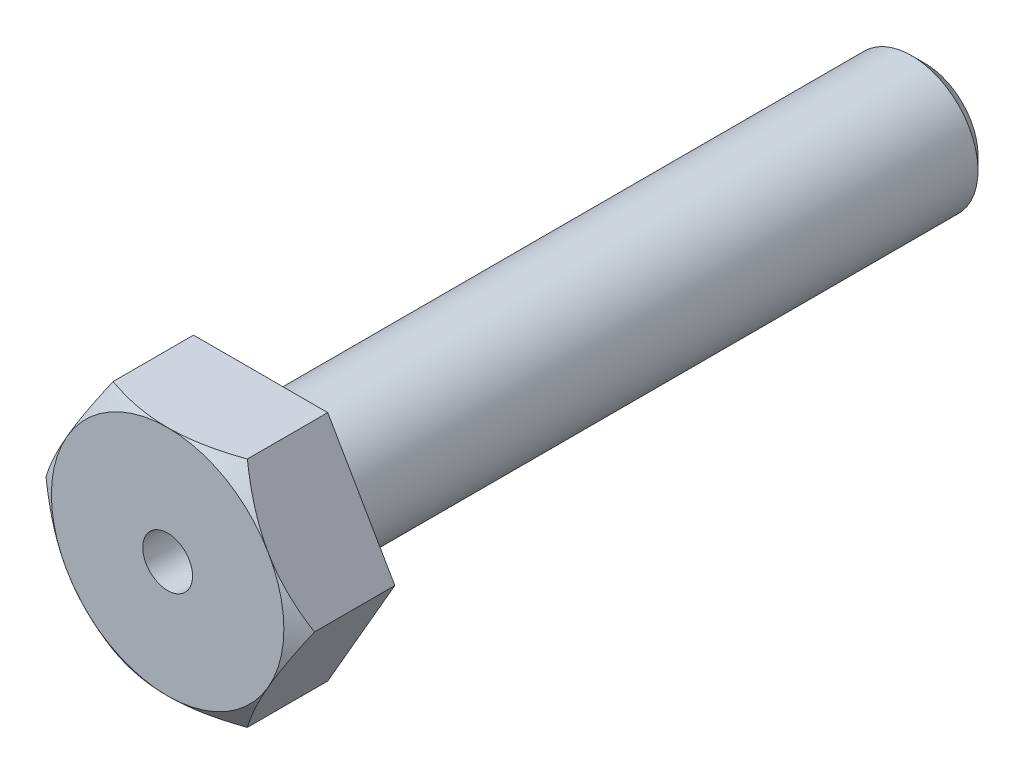
from build123d import *

# Parameters (mm, degrees)
BOSS_EXTRUDE1_START = -2.8
SKETCH4_R           = 0.75
BOSS_EXTRUDE1_DEPTH = 2.8
SKETCH5_R           = 4.582903769
SKETCH5_R_2         = 3.5
CUT_EXTRUDE1_DEPTH  = 1
CUT_EXTRUDE1_DRAFT  = -55
CHAMFER1_SIZE       = 0.4


with BuildPart() as part:
    # Sketch3 → Revolve1 (revolve)
    with BuildSketch(Plane(origin=(0, 0, 0), x_dir=(0, 0, -1), z_dir=(1, 0, 0)), mode=Mode.PRIVATE) as revolve1_sk:
        Polygon((0, 2), (-2.8, 2), (-2.8, 0.75), (20, 0.75), (20, 2), align=None)
    revolve(revolve1_sk.sketch.rotate(Axis((0, 0, 2.8), (0, 0, -1)), 180), axis=Axis((0, 0, 2.8), (0, 0, -1)))

    # Sketch4 → Boss-Extrude1 (add)
    with BuildSketch(Plane.XY.offset(2.8).offset(BOSS_EXTRUDE1_START)):
        Polygon((2.020725942, 3.5), (-2.020725942, 3.5), (-4.041451884, 0), (-2.020725942, -3.5), (2.020725942, -3.5), (4.041451884, 0), align=None)
        with Locations(Location((0, 0, 0), (0, 0, 270))):
            Circle(SKETCH4_R, mode=Mode.SUBTRACT)
    extrude(amount=BOSS_EXTRUDE1_DEPTH)


with BuildPart() as cut_extrude1_tool:
    # Sketch5 → Cut-Extrude1 (with draft: the straight prism first)
    with BuildSketch(Plane.XY.offset(2.8)):
        Circle(SKETCH5_R)
        Circle(SKETCH5_R_2, mode=Mode.SUBTRACT)
    extrude(amount=-CUT_EXTRUDE1_DEPTH)
    # Cut-Extrude1: the draft: its side faces are tilted about the plane it starts from
    cut_extrude1_sides = [cut_extrude1_tool.faces().sort_by_distance(p)[0] for p in [
        (-4.582903769, 0, 2.3),
        (-3.5, 0, 2.3),
    ]]
    draft(cut_extrude1_sides, Plane.XY.offset(2.8), CUT_EXTRUDE1_DRAFT)


with BuildPart() as part_1:
    add(part.part)

    # Cut-Extrude1: cut by cut_extrude1_tool
    add(cut_extrude1_tool.part, mode=Mode.SUBTRACT)

    # Chamfer1
    chamfer1_edges = [part_1.edges().sort_by_distance(p)[0] for p in [
        (0, 2, -20),
    ]]
    chamfer(chamfer1_edges, length=CHAMFER1_SIZE)


solid = part_1.part
